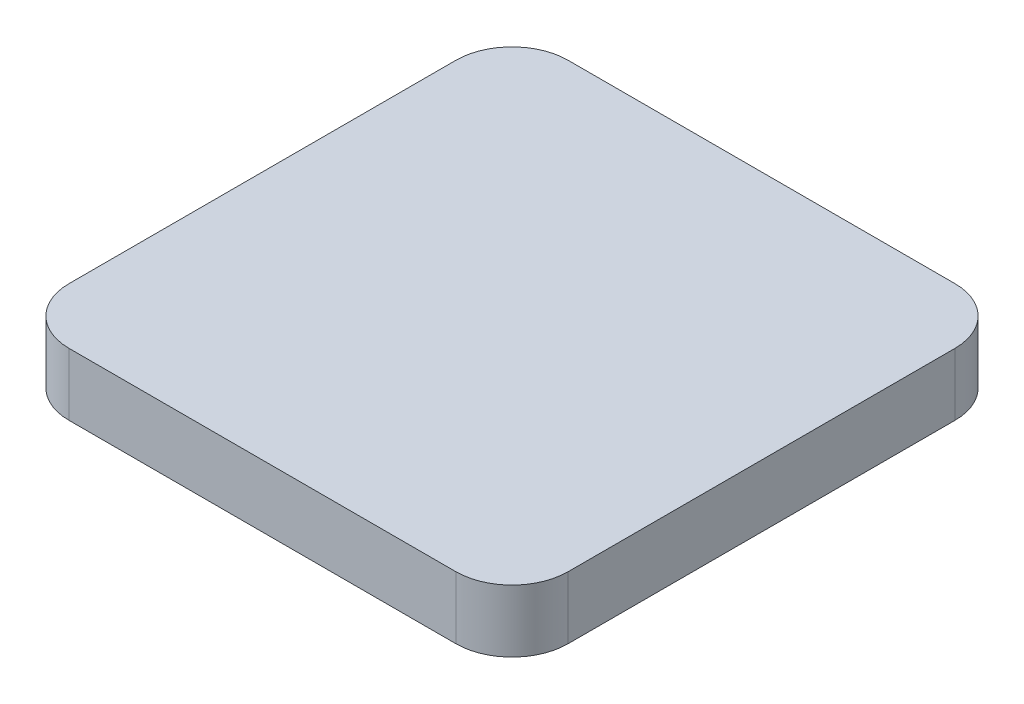
SolidWorks part; units mm, degrees
material "黑色POM "
ref_plane "前基準面" through (0, 0, 0) normal (0, 0, 1) x (1, 0, 0)
ref_plane "上基準面" through (0, 0, 0) normal (0, 1, 0) x (1, 0, 0)
ref_plane "右基準面" through (0, 0, 0) normal (1, 0, 0) x (0, 0, -1)
sketch "草图1" plane through (0, 0, 0) normal (0, 1, 0) x (1, 0, 0)
  line L1 (-20, -20) -> (20, -20)
  line L2 (-20, -20) -> (-20, 20)
  line L3 (-20, 20) -> (20, 20)
  line L4 (20, -20) -> (20, 20)
  line L5 (-20, -20) -> (20, 20) construction
  line L6 (-20, 20) -> (20, -20) construction
  point P0 (0, 0)
  dimension "D1" = 40
  dimension "D2" = 40
extrude "凸台-拉伸1" add sketch "草图1" along normal mid plane 5
fillet "圆角1" radius 4.5 4 edges at (20, 0, -20) (20, 0, 20) (-20, 0, -20) (-20, 0, 20)
